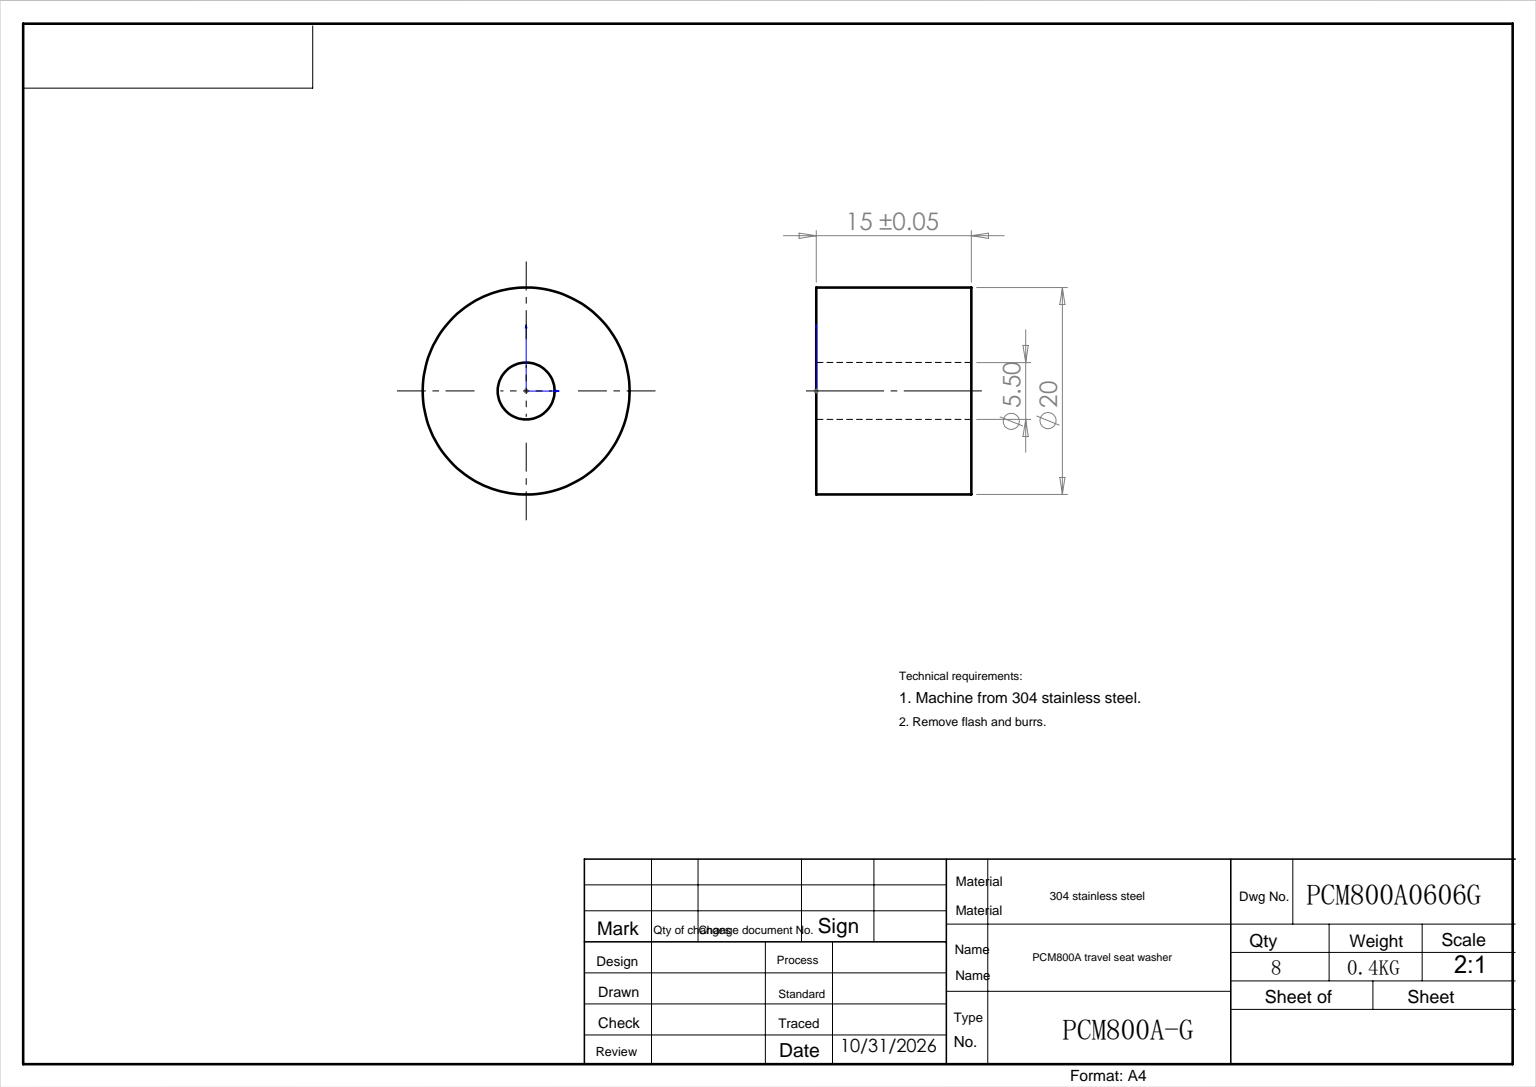
from build123d import *

# Parameters (mm, degrees)
SKETCH_1_R      = 10
SKETCH_1_R_2    = 2.75
EXTRUDE_1_DEPTH = 15


with BuildPart() as part:
    # 草图1 → 凸台-拉伸1 (new body)
    with BuildSketch(Plane.XY):
        Circle(SKETCH_1_R)
        Circle(SKETCH_1_R_2, mode=Mode.SUBTRACT)
    extrude(amount=EXTRUDE_1_DEPTH)


solid = part.part
